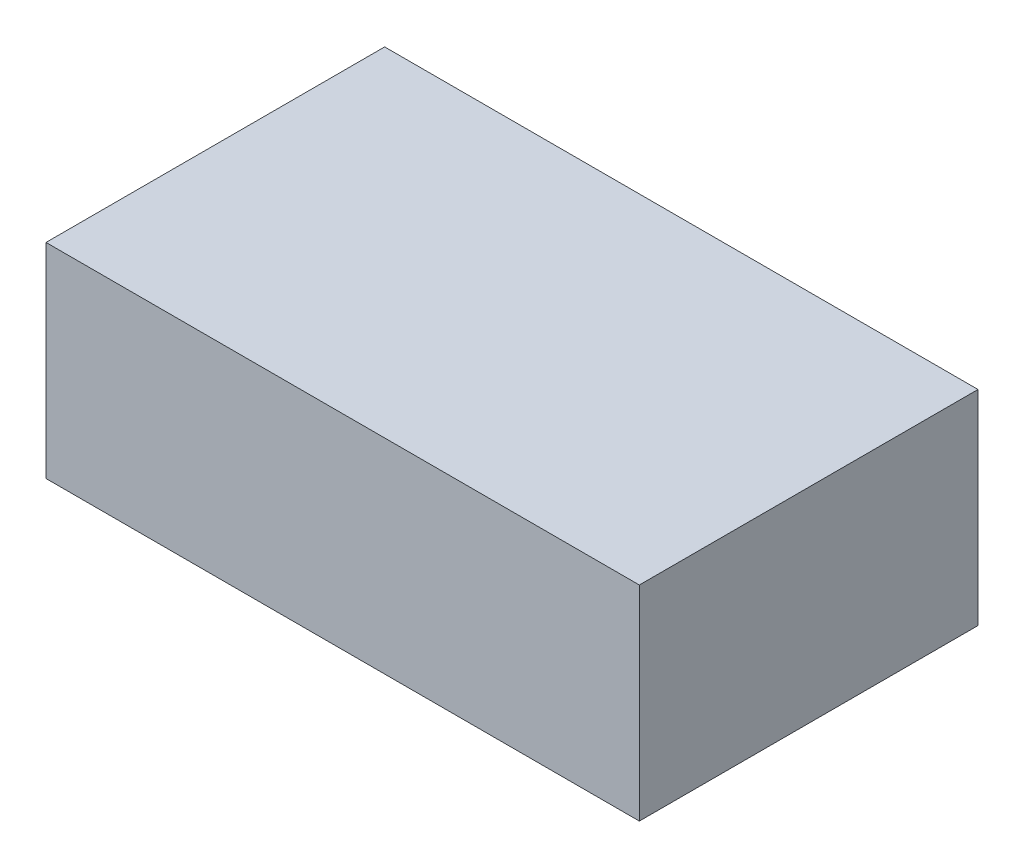
from build123d import *

# Parameters (mm, degrees)
SKETCH_1_W               = 6500
SKETCH_1_H               = 3710
EXTRUDE_1_DEPTH          = 2240
CUT_EXTRUDE_1_DEPTH      = 3220
CUT_EXTRUDE_1_DEPTH_BACK = 3220
SKETCH_2_W               = 3650
SKETCH_2_H               = 2180


with BuildPart() as part:
    # 草图1 → 凸台-拉伸1 (new body)
    with BuildSketch(Plane(origin=(0, 0, 0), x_dir=(1, 0, 0), z_dir=(0, 1, 0))):
        Rectangle(SKETCH_1_W, SKETCH_1_H)
    extrude(amount=EXTRUDE_1_DEPTH)

    # 草图2 → 切除-拉伸1 (cut, two sides: drawn at the far end of the back side and taken through both)
    with BuildSketch(Plane(origin=(0, 0, 0), x_dir=(0, 0, -1), z_dir=(1, 0, 0)).offset(-CUT_EXTRUDE_1_DEPTH_BACK)):
        with Locations((0, 1120)):
            Rectangle(SKETCH_2_W, SKETCH_2_H)
    extrude(amount=CUT_EXTRUDE_1_DEPTH + CUT_EXTRUDE_1_DEPTH_BACK, mode=Mode.SUBTRACT)


solid = part.part
